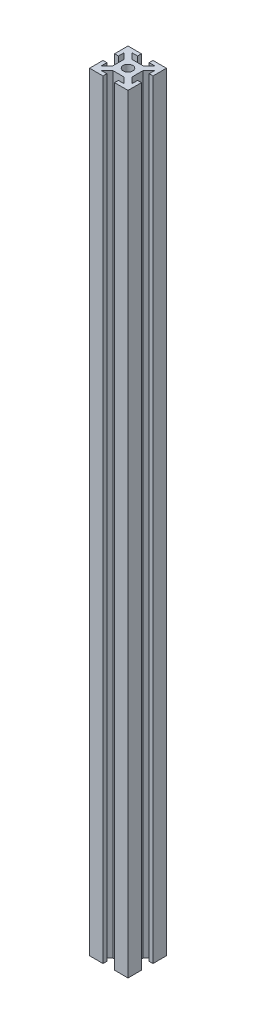
from build123d import *

# Parameters (mm, degrees)
SKETCH1_R           = 5
BOSS_EXTRUDE1_DEPTH = 800


with BuildPart() as part:
    # Sketch1 → Boss-Extrude1 (new body)
    with BuildSketch(Plane(origin=(0, 0, 0), x_dir=(1, 0, 0), z_dir=(0, 1, 0))):
        Polygon((-6, 20), (-6, 16), (-11.757359313, 16), (-5.757359313, 10), (5.757359313, 10), (11.757359313, 16), (6, 16), (6, 20), (20, 20), (20, 6), (16, 6), (16, 11.757359313), (10, 5.757359313), (10, -5.757359313), (16, -11.757359313), (16, -6), (20, -6), (20, -20), (6, -20), (6, -16), (11.757359313, -16), (5.757359313, -10), (-5.757359313, -10), (-11.757359313, -16), (-6, -16), (-6, -20), (-20, -20), (-20, -6), (-16, -6), (-16, -11.757359313), (-10, -5.757359313), (-10, 5.757359313), (-16, 11.757359313), (-16, 6), (-20, 6), (-20, 20), align=None)
        with Locations(Location((0, 0, 0), (0, 0, 270))):
            Circle(SKETCH1_R, mode=Mode.SUBTRACT)
    extrude(amount=BOSS_EXTRUDE1_DEPTH)


solid = part.part
